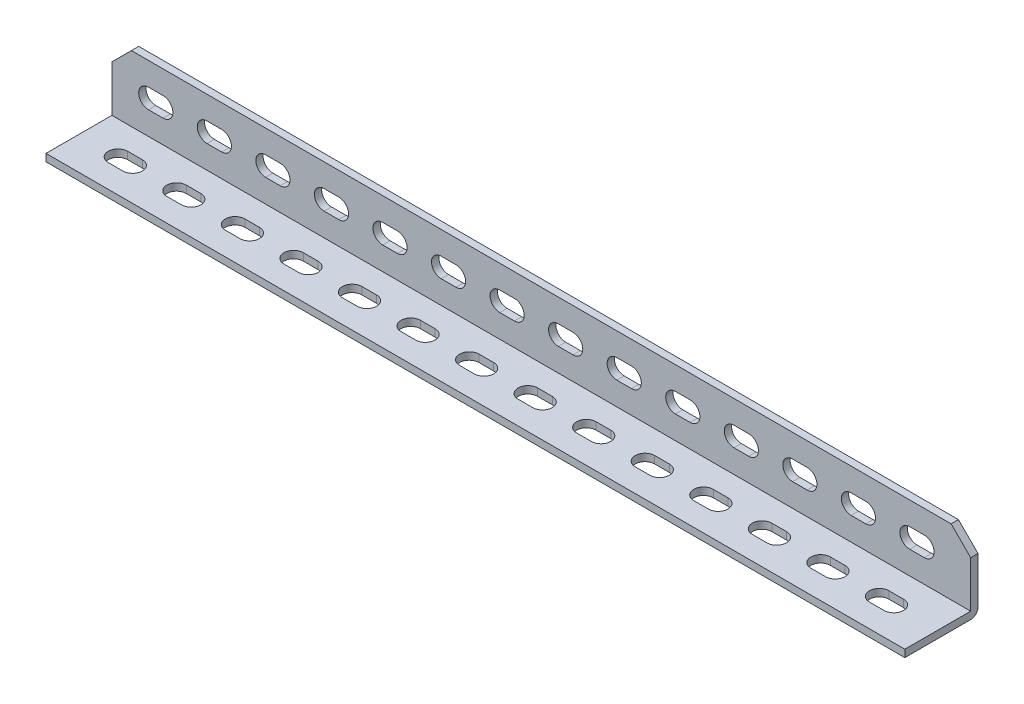
SolidWorks part; units mm, degrees
material "SPCC"
ref_plane "Front Plane" through (0, 0, 0) normal (0, 0, 1) x (1, 0, 0)
ref_plane "Top Plane" through (0, 0, 0) normal (0, 1, 0) x (1, 0, 0)
ref_plane "Right Plane" through (0, 0, 0) normal (1, 0, 0) x (0, 0, -1)
other "Configuration Table"
sketch "Sketch1" plane through (0, 0, 0) normal (0, 0, 1) x (1, 0, 0)
  line L0 (-69.244, -28.9983) -> (282.756, -28.9983)
  line L1 (-69.244, -28.9983) -> (-69.244, -1.9983)
  line L2 (-69.244, -1.9983) -> (282.756, -1.9983)
  line L3 (282.756, -1.9983) -> (282.756, -28.9983)
  dimension "D1" = 27
  dimension "D2" = 352
extrude "Boss-Extrude1" add sketch "Sketch1" along normal blind 3
sketch "Sketch3" plane through (0, -28.9983, 0) normal (0, -1, 0) x (1, 0, 0)
  line L0 (-69.244, 0) -> (-69.244, 30)
  line L1 (-69.244, 30) -> (282.756, 30)
  line L2 (282.756, 30) -> (282.756, 0)
  line L3 (282.756, 0) -> (-69.244, 0)
  dimension "D1" = 30
extrude "Boss-Extrude2" add sketch "Sketch3" along normal blind 3
fillet "Fillet1" radius 3 1 edges at (106.756, -31.9983, 0)
sketch "Sketch4" plane through (0, -28.9983, 0) normal (0, 1, 0) x (1, 0, 0)
  line L0 (-69.244, -16.5) -> (282.756, -16.5) construction
  line L1 (-69.244, -30) -> (-69.244, -3) construction
  line L2 (282.756, -3) -> (282.756, -30) construction
  line L3 (-53.244, -12.5) -> (-53.244, -20.5) construction
  line L4 (-53.244, -12.5) -> (-47.244, -12.5)
  line L5 (-47.244, -12.5) -> (-47.244, -20.5) construction
  line L6 (-53.244, -20.5) -> (-47.244, -20.5)
  line L7 (-29.244, -12.5) -> (-23.244, -12.5)
  line L8 (-29.244, -20.5) -> (-23.244, -20.5)
  line L9 (-5.244, -12.5) -> (0.756, -12.5)
  line L10 (-5.244, -20.5) -> (0.756, -20.5)
  line L11 (18.756, -12.5) -> (24.756, -12.5)
  line L12 (18.756, -20.5) -> (24.756, -20.5)
  line L13 (42.756, -12.5) -> (48.756, -12.5)
  line L14 (42.756, -20.5) -> (48.756, -20.5)
  line L15 (66.756, -12.5) -> (72.756, -12.5)
  line L16 (66.756, -20.5) -> (72.756, -20.5)
  line L17 (90.756, -12.5) -> (96.756, -12.5)
  line L18 (90.756, -20.5) -> (96.756, -20.5)
  line L19 (114.756, -12.5) -> (120.756, -12.5)
  line L20 (114.756, -20.5) -> (120.756, -20.5)
  line L21 (138.756, -12.5) -> (144.756, -12.5)
  line L22 (138.756, -20.5) -> (144.756, -20.5)
  line L23 (162.756, -12.5) -> (168.756, -12.5)
  line L24 (162.756, -20.5) -> (168.756, -20.5)
  line L25 (186.756, -12.5) -> (192.756, -12.5)
  line L26 (186.756, -20.5) -> (192.756, -20.5)
  line L27 (210.756, -12.5) -> (216.756, -12.5)
  line L28 (210.756, -20.5) -> (216.756, -20.5)
  line L29 (234.756, -12.5) -> (240.756, -12.5)
  line L30 (234.756, -20.5) -> (240.756, -20.5)
  line L31 (258.756, -12.5) -> (264.756, -12.5)
  line L32 (258.756, -20.5) -> (264.756, -20.5)
  line L45 (306.756, -12.5) -> (312.756, -12.5) [skipped]
  line L46 (306.756, -20.5) -> (312.756, -20.5) [skipped]
  line L47 (330.756, -12.5) -> (336.756, -12.5) [skipped]
  line L48 (330.756, -20.5) -> (336.756, -20.5) [skipped]
  line L49 (354.756, -12.5) -> (360.756, -12.5) [skipped]
  line L50 (354.756, -20.5) -> (360.756, -20.5) [skipped]
  line L51 (378.756, -12.5) -> (384.756, -12.5) [skipped]
  line L52 (378.756, -20.5) -> (384.756, -20.5) [skipped]
  line L53 (402.756, -12.5) -> (408.756, -12.5) [skipped]
  line L54 (402.756, -20.5) -> (408.756, -20.5) [skipped]
  line L55 (282.756, -12.5) -> (288.756, -12.5) [skipped]
  line L56 (282.756, -20.5) -> (288.756, -20.5) [skipped]
  arc A0 (-53.244, -12.5) -> (-53.244, -20.5) centre (-53.244, -16.5) ccw
  arc A1 (-47.244, -20.5) -> (-47.244, -12.5) centre (-47.244, -16.5) ccw
  arc A2 (-29.244, -12.5) -> (-29.244, -20.5) centre (-29.244, -16.5) ccw
  arc A3 (-23.244, -20.5) -> (-23.244, -12.5) centre (-23.244, -16.5) ccw
  arc A4 (-5.244, -12.5) -> (-5.244, -20.5) centre (-5.244, -16.5) ccw
  arc A5 (0.756, -20.5) -> (0.756, -12.5) centre (0.756, -16.5) ccw
  arc A6 (18.756, -12.5) -> (18.756, -20.5) centre (18.756, -16.5) ccw
  arc A7 (24.756, -20.5) -> (24.756, -12.5) centre (24.756, -16.5) ccw
  arc A8 (42.756, -12.5) -> (42.756, -20.5) centre (42.756, -16.5) ccw
  arc A9 (48.756, -20.5) -> (48.756, -12.5) centre (48.756, -16.5) ccw
  arc A10 (66.756, -12.5) -> (66.756, -20.5) centre (66.756, -16.5) ccw
  arc A11 (72.756, -20.5) -> (72.756, -12.5) centre (72.756, -16.5) ccw
  arc A12 (90.756, -12.5) -> (90.756, -20.5) centre (90.756, -16.5) ccw
  arc A13 (96.756, -20.5) -> (96.756, -12.5) centre (96.756, -16.5) ccw
  arc A14 (114.756, -12.5) -> (114.756, -20.5) centre (114.756, -16.5) ccw
  arc A15 (120.756, -20.5) -> (120.756, -12.5) centre (120.756, -16.5) ccw
  arc A16 (138.756, -12.5) -> (138.756, -20.5) centre (138.756, -16.5) ccw
  arc A17 (144.756, -20.5) -> (144.756, -12.5) centre (144.756, -16.5) ccw
  arc A18 (162.756, -12.5) -> (162.756, -20.5) centre (162.756, -16.5) ccw
  arc A19 (168.756, -20.5) -> (168.756, -12.5) centre (168.756, -16.5) ccw
  arc A20 (186.756, -12.5) -> (186.756, -20.5) centre (186.756, -16.5) ccw
  arc A21 (192.756, -20.5) -> (192.756, -12.5) centre (192.756, -16.5) ccw
  arc A22 (210.756, -12.5) -> (210.756, -20.5) centre (210.756, -16.5) ccw
  arc A23 (216.756, -20.5) -> (216.756, -12.5) centre (216.756, -16.5) ccw
  arc A24 (234.756, -12.5) -> (234.756, -20.5) centre (234.756, -16.5) ccw
  arc A25 (240.756, -20.5) -> (240.756, -12.5) centre (240.756, -16.5) ccw
  arc A26 (258.756, -12.5) -> (258.756, -20.5) centre (258.756, -16.5) ccw
  arc A27 (264.756, -20.5) -> (264.756, -12.5) centre (264.756, -16.5) ccw
  arc A40 (288.756, -20.5) -> (288.756, -12.5) centre (288.756, -16.5) ccw [skipped]
  arc A41 (306.756, -12.5) -> (306.756, -20.5) centre (306.756, -16.5) ccw [skipped]
  arc A42 (312.756, -20.5) -> (312.756, -12.5) centre (312.756, -16.5) ccw [skipped]
  arc A43 (330.756, -12.5) -> (330.756, -20.5) centre (330.756, -16.5) ccw [skipped]
  arc A44 (336.756, -20.5) -> (336.756, -12.5) centre (336.756, -16.5) ccw [skipped]
  arc A45 (354.756, -12.5) -> (354.756, -20.5) centre (354.756, -16.5) ccw [skipped]
  arc A46 (360.756, -20.5) -> (360.756, -12.5) centre (360.756, -16.5) ccw [skipped]
  arc A47 (378.756, -12.5) -> (378.756, -20.5) centre (378.756, -16.5) ccw [skipped]
  arc A48 (384.756, -20.5) -> (384.756, -12.5) centre (384.756, -16.5) ccw [skipped]
  arc A49 (402.756, -12.5) -> (402.756, -20.5) centre (402.756, -16.5) ccw [skipped]
  arc A50 (408.756, -20.5) -> (408.756, -12.5) centre (408.756, -16.5) ccw [skipped]
  arc A51 (282.756, -12.5) -> (282.756, -20.5) centre (282.756, -16.5) ccw [skipped]
  point P12 (-57.244, -16.5)
  dimension "D1" = 8
  dimension "D3" = 6
  dimension "D2" = 12
  dimension "D4" = 20
extrude "Cut-Extrude1" cut sketch "Sketch4" against normal blind 3
sketch "Sketch5" plane through (0, 0, 3) normal (0, 0, 1) x (1, 0, 0)
  line L0 (-69.244, -15.4983) -> (282.756, -15.4983) construction
  line L1 (-69.244, -28.9983) -> (-69.244, -1.9983) construction
  line L2 (282.756, -1.9983) -> (282.756, -28.9983) construction
  line L3 (-54.244, -11.4983) -> (-54.244, -19.4983) construction
  line L4 (-54.244, -11.4983) -> (-48.244, -11.4983)
  line L5 (-54.244, -19.4983) -> (-48.244, -19.4983)
  line L6 (-30.244, -11.4983) -> (-24.244, -11.4983)
  line L7 (-30.244, -19.4983) -> (-24.244, -19.4983)
  line L8 (-6.244, -11.4983) -> (-0.244, -11.4983)
  line L9 (-6.244, -19.4983) -> (-0.244, -19.4983)
  line L10 (17.756, -11.4983) -> (23.756, -11.4983)
  line L11 (17.756, -19.4983) -> (23.756, -19.4983)
  line L12 (41.756, -11.4983) -> (47.756, -11.4983)
  line L13 (41.756, -19.4983) -> (47.756, -19.4983)
  line L14 (65.756, -11.4983) -> (71.756, -11.4983)
  line L15 (65.756, -19.4983) -> (71.756, -19.4983)
  line L16 (89.756, -11.4983) -> (95.756, -11.4983)
  line L17 (89.756, -19.4983) -> (95.756, -19.4983)
  line L18 (113.756, -11.4983) -> (119.756, -11.4983)
  line L19 (113.756, -19.4983) -> (119.756, -19.4983)
  line L20 (137.756, -11.4983) -> (143.756, -11.4983)
  line L21 (137.756, -19.4983) -> (143.756, -19.4983)
  line L22 (161.756, -11.4983) -> (167.756, -11.4983)
  line L23 (161.756, -19.4983) -> (167.756, -19.4983)
  line L24 (185.756, -11.4983) -> (191.756, -11.4983)
  line L25 (185.756, -19.4983) -> (191.756, -19.4983)
  line L26 (209.756, -11.4983) -> (215.756, -11.4983)
  line L27 (209.756, -19.4983) -> (215.756, -19.4983)
  line L28 (233.756, -11.4983) -> (239.756, -11.4983)
  line L29 (233.756, -19.4983) -> (239.756, -19.4983)
  line L30 (257.756, -11.4983) -> (263.756, -11.4983)
  line L31 (257.756, -19.4983) -> (263.756, -19.4983)
  line L44 (281.756, -11.4983) -> (287.756, -11.4983) [skipped]
  line L45 (281.756, -19.4983) -> (287.756, -19.4983) [skipped]
  line L46 (305.756, -11.4983) -> (311.756, -11.4983) [skipped]
  line L47 (305.756, -19.4983) -> (311.756, -19.4983) [skipped]
  line L48 (329.756, -11.4983) -> (335.756, -11.4983) [skipped]
  line L49 (329.756, -19.4983) -> (335.756, -19.4983) [skipped]
  line L50 (353.756, -11.4983) -> (359.756, -11.4983) [skipped]
  line L51 (353.756, -19.4983) -> (359.756, -19.4983) [skipped]
  line L52 (377.756, -11.4983) -> (383.756, -11.4983) [skipped]
  line L53 (377.756, -19.4983) -> (383.756, -19.4983) [skipped]
  line L54 (401.756, -11.4983) -> (407.756, -11.4983) [skipped]
  line L55 (401.756, -19.4983) -> (407.756, -19.4983) [skipped]
  arc A0 (-54.244, -11.4983) -> (-54.244, -19.4983) centre (-54.244, -15.4983) ccw
  arc A1 (-48.244, -19.4983) -> (-48.244, -11.4983) centre (-48.244, -15.4983) ccw
  arc A2 (-30.244, -11.4983) -> (-30.244, -19.4983) centre (-30.244, -15.4983) ccw
  arc A3 (-24.244, -19.4983) -> (-24.244, -11.4983) centre (-24.244, -15.4983) ccw
  arc A4 (-6.244, -11.4983) -> (-6.244, -19.4983) centre (-6.244, -15.4983) ccw
  arc A5 (-0.244, -19.4983) -> (-0.244, -11.4983) centre (-0.244, -15.4983) ccw
  arc A6 (17.756, -11.4983) -> (17.756, -19.4983) centre (17.756, -15.4983) ccw
  arc A7 (23.756, -19.4983) -> (23.756, -11.4983) centre (23.756, -15.4983) ccw
  arc A8 (41.756, -11.4983) -> (41.756, -19.4983) centre (41.756, -15.4983) ccw
  arc A9 (47.756, -19.4983) -> (47.756, -11.4983) centre (47.756, -15.4983) ccw
  arc A10 (65.756, -11.4983) -> (65.756, -19.4983) centre (65.756, -15.4983) ccw
  arc A11 (71.756, -19.4983) -> (71.756, -11.4983) centre (71.756, -15.4983) ccw
  arc A12 (89.756, -11.4983) -> (89.756, -19.4983) centre (89.756, -15.4983) ccw
  arc A13 (95.756, -19.4983) -> (95.756, -11.4983) centre (95.756, -15.4983) ccw
  arc A14 (113.756, -11.4983) -> (113.756, -19.4983) centre (113.756, -15.4983) ccw
  arc A15 (119.756, -19.4983) -> (119.756, -11.4983) centre (119.756, -15.4983) ccw
  arc A16 (137.756, -11.4983) -> (137.756, -19.4983) centre (137.756, -15.4983) ccw
  arc A17 (143.756, -19.4983) -> (143.756, -11.4983) centre (143.756, -15.4983) ccw
  arc A18 (161.756, -11.4983) -> (161.756, -19.4983) centre (161.756, -15.4983) ccw
  arc A19 (167.756, -19.4983) -> (167.756, -11.4983) centre (167.756, -15.4983) ccw
  arc A20 (185.756, -11.4983) -> (185.756, -19.4983) centre (185.756, -15.4983) ccw
  arc A21 (191.756, -19.4983) -> (191.756, -11.4983) centre (191.756, -15.4983) ccw
  arc A22 (209.756, -11.4983) -> (209.756, -19.4983) centre (209.756, -15.4983) ccw
  arc A23 (215.756, -19.4983) -> (215.756, -11.4983) centre (215.756, -15.4983) ccw
  arc A24 (233.756, -11.4983) -> (233.756, -19.4983) centre (233.756, -15.4983) ccw
  arc A25 (239.756, -19.4983) -> (239.756, -11.4983) centre (239.756, -15.4983) ccw
  arc A26 (257.756, -11.4983) -> (257.756, -19.4983) centre (257.756, -15.4983) ccw
  arc A27 (263.756, -19.4983) -> (263.756, -11.4983) centre (263.756, -15.4983) ccw
  arc A40 (281.756, -11.4983) -> (281.756, -19.4983) centre (281.756, -15.4983) ccw [skipped]
  arc A41 (287.756, -19.4983) -> (287.756, -11.4983) centre (287.756, -15.4983) ccw [skipped]
  arc A42 (305.756, -11.4983) -> (305.756, -19.4983) centre (305.756, -15.4983) ccw [skipped]
  arc A43 (311.756, -19.4983) -> (311.756, -11.4983) centre (311.756, -15.4983) ccw [skipped]
  arc A44 (329.756, -11.4983) -> (329.756, -19.4983) centre (329.756, -15.4983) ccw [skipped]
  arc A45 (335.756, -19.4983) -> (335.756, -11.4983) centre (335.756, -15.4983) ccw [skipped]
  arc A46 (353.756, -11.4983) -> (353.756, -19.4983) centre (353.756, -15.4983) ccw [skipped]
  arc A47 (359.756, -19.4983) -> (359.756, -11.4983) centre (359.756, -15.4983) ccw [skipped]
  arc A48 (377.756, -11.4983) -> (377.756, -19.4983) centre (377.756, -15.4983) ccw [skipped]
  arc A49 (383.756, -19.4983) -> (383.756, -11.4983) centre (383.756, -15.4983) ccw [skipped]
  arc A50 (401.756, -11.4983) -> (401.756, -19.4983) centre (401.756, -15.4983) ccw [skipped]
  arc A51 (407.756, -19.4983) -> (407.756, -11.4983) centre (407.756, -15.4983) ccw [skipped]
  dimension "D1" = 8
  dimension "D2" = 15
  dimension "D4" = 20
  dimension "D3" = 6
extrude "Cut-Extrude2" cut sketch "Sketch5" against normal blind 3
sketch "Sketch6" plane through (0, 0, 3) normal (0, 0, 1) x (1, 0, 0)
  line L0 (-69.244, -7.9983) -> (-69.244, -9.9983)
  line L4 (-69.244, -1.9983) -> (282.756, -1.9983) construction
  line L5 (274.756, -1.9983) -> (282.756, -1.9983)
  line L6 (282.756, -1.9983) -> (282.756, -9.9983)
  line L7 (-69.244, -28.9983) -> (-69.244, -1.9983) construction
  line L12 (-63.244, -1.9983) -> (-93.244, -31.9983) construction
  line L13 (-69.244, -9.9983) -> (-69.244, -1.9983)
  line L14 (-69.244, -1.9983) -> (-61.244, -1.9983)
  line L15 (-61.244, -1.9983) -> (-69.244, -9.9983)
  line L18 (282.756, -9.9983) -> (282.756, -1.9983)
  line L19 (282.756, -1.9983) -> (274.756, -1.9983)
  line L20 (274.756, -1.9983) -> (282.756, -9.9983)
  dimension "D1" = 8
  dimension "D2" = 8
  dimension "D3" = 8
  dimension "D4" = 8
extrude "Cut-Extrude4" cut sketch "Sketch6" against normal blind 3 contours L15 L14 L13 L0 | L5 L20 L6
